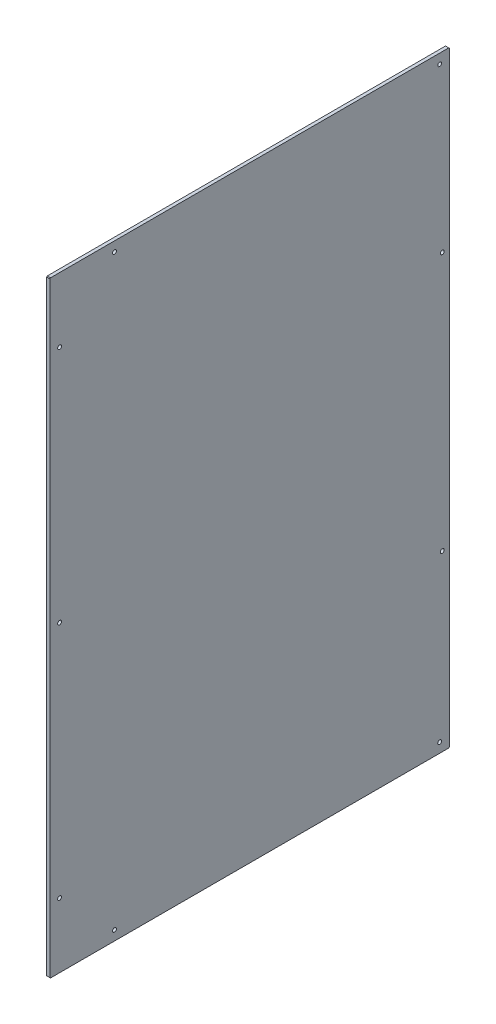
from build123d import *

# Parameters (mm, degrees)
SKETCH_1_W          = 618
SKETCH_1_H          = 938
EXTRUDE_1_DEPTH     = 5
CHAMFER_1_SIZE      = 1
SKETCH_2_R          = 3
CUT_EXTRUDE_1_DEPTH = 562.664490599


with BuildPart() as part:
    # 草图1 → 凸台-拉伸1 (new body)
    with BuildSketch(Plane(origin=(0, 0, 0), x_dir=(0, 0, -1), z_dir=(1, 0, 0))):
        Rectangle(SKETCH_1_W, SKETCH_1_H)
    extrude(amount=EXTRUDE_1_DEPTH)

    # 倒角1
    chamfer_1_edges = [part.edges().sort_by_distance(p)[0] for p in [
        (2.5, 469, 309),
        (2.5, 469, -309),
        (2.5, -469, -309),
        (2.5, -469, 309),
    ]]
    chamfer(chamfer_1_edges, length=CHAMFER_1_SIZE)

    # 草图2 → 切除-拉伸1 (cut, through all)
    with BuildSketch(Plane.ZY):
        with Locations((-294, 454)):
            Circle(SKETCH_2_R)
        with Locations(Location((-294, -454, 0), (0, 0, 180))):
            Circle(SKETCH_2_R)
        with Locations((209, 454)):
            Circle(SKETCH_2_R)
        with Locations((294, 369)):
            Circle(SKETCH_2_R)
        with Locations((294, -369)):
            Circle(SKETCH_2_R)
        with Locations((209, -454)):
            Circle(SKETCH_2_R)
        with Locations((294, 0)):
            Circle(SKETCH_2_R)
        with Locations((-298, 200)):
            Circle(SKETCH_2_R)
        with Locations((-298, -200)):
            Circle(SKETCH_2_R)
    extrude(amount=-CUT_EXTRUDE_1_DEPTH, mode=Mode.SUBTRACT)


solid = part.part
